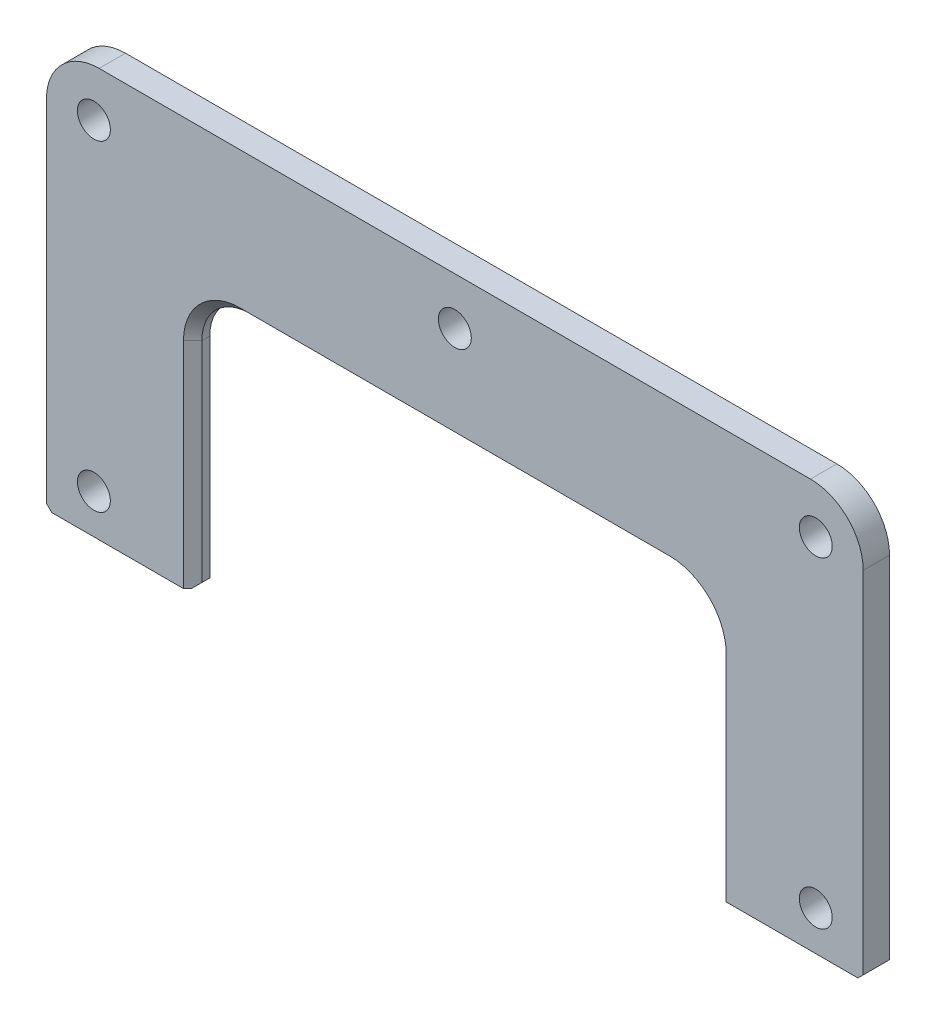
SolidWorks part; units mm, degrees
material "耐油橡胶板 3002"
ref_plane "前视基准面" through (0, 0, 0) normal (0, 0, 1) x (1, 0, 0)
ref_plane "上视基准面" through (0, 0, 0) normal (0, 1, 0) x (1, 0, 0)
ref_plane "右视基准面" through (0, 0, 0) normal (1, 0, 0) x (0, 0, -1)
sketch "草图1" plane through (0, 0, 0) normal (0, 0, 1) x (1, 0, 0)
  line L0 (-155, 0) -> (-99.5, 0)
  line L1 (-81.5, 99.5) -> (81.5, 99.5)
  line L2 (-99.5, 81.5) -> (-99.5, 2.5)
  line L3 (-81.5, -99.5) -> (81.5, -99.5) construction
  line L4 (99.5, 81.5) -> (99.5, 2.5)
  line L5 (-99.5, 99.5) -> (99.5, -99.5) construction
  line L6 (-99.5, -99.5) -> (99.5, 99.5) construction
  line L7 (-135, -155) -> (135, -155) construction
  line L8 (-155, -135) -> (-155, 0) construction
  line L9 (-135, 155) -> (135, 155)
  line L10 (155, -135) -> (155, 0) construction
  line L11 (-155, -155) -> (155, 155) construction
  line L12 (-155, 155) -> (155, -155) construction
  line L13 (-155, 2.5) -> (-99.5, 2.5) construction
  line L14 (-99.5, 2.5) -> (99.5, 2.5) construction
  line L15 (99.5, 2.5) -> (155, 2.5) construction
  line L16 (-155, 2.5) -> (-155, 135)
  line L17 (-99.5, 0) -> (-99.5, -81.5) construction
  line L18 (99.5, 0) -> (99.5, -81.5) construction
  line L19 (155, 2.5) -> (155, 135)
  line L20 (-155, 2.5) -> (-155, 0)
  line L21 (-99.5, 2.5) -> (-99.5, 0)
  line L22 (99.5, 2.5) -> (99.5, 0)
  line L23 (155, 2.5) -> (155, 0)
  line L24 (99.5, 0) -> (155, 0)
  arc A0 (-81.5, -99.5) -> (-99.5, -81.5) centre (-81.5, -81.5) cw construction
  arc A1 (81.5, -99.5) -> (99.5, -81.5) centre (81.5, -81.5) ccw construction
  arc A2 (99.5, 81.5) -> (81.5, 99.5) centre (81.5, 81.5) ccw
  arc A3 (-99.5, 81.5) -> (-81.5, 99.5) centre (-81.5, 81.5) cw
  arc A4 (135, -155) -> (155, -135) centre (135, -135) ccw construction
  arc A5 (-135, -155) -> (-155, -135) centre (-135, -135) cw construction
  arc A6 (155, 135) -> (135, 155) centre (135, 135) ccw
  arc A7 (-155, 135) -> (-135, 155) centre (-135, 135) cw
  point P0 (0, 0)
  point P18 (0, 0)
  dimension "D3" = 18
  dimension "D6" = 20
  dimension "D1" = 199
  dimension "D2" = 199
  dimension "D4" = 310
  dimension "D5" = 310
  dimension "D7" = 2.5
extrude "凸台-拉伸1" add sketch "草图1" along normal blind 10
sketch "草图2" plane through (0, 0, 10) normal (0, 0, 1) x (1, 0, 0)
  line L0 (135, 155) -> (-135, 155) construction
  line L1 (-137, -137) -> (137, -137) construction
  line L2 (-137, -137) -> (-137, 137) construction
  line L3 (-137, 137) -> (137, 137) construction
  line L4 (137, -137) -> (137, 137) construction
  line L5 (-137, -137) -> (137, 137) construction
  line L6 (-137, 137) -> (137, -137) construction
  line L8 (-137, 0) -> (0, 0) construction
  line L9 (0, 0) -> (0, 137) construction
  line L10 (155, 0) -> (155, 135) construction
  circle A0 centre (0, 137) radius 6.25
  circle A1 centre (0, -137) radius 6.25
  circle A2 centre (137, 0) radius 6.25 construction
  circle A3 centre (-137, 0) radius 6.25 construction
  circle A4 centre (-137, 137) radius 6.25
  circle A5 centre (137, 137) radius 6.25
  circle A6 centre (-137, -137) radius 6.25
  circle A7 centre (137, -137) radius 6.25
  circle A8 centre (-137, 15) radius 6.25
  circle A9 centre (-137, -15) radius 6.25
  circle A10 centre (137, -15) radius 6.25
  circle A11 centre (137, 15) radius 6.25
  point P0 (0, 0)
  dimension "D3" = 12.5
  dimension "D1" = 18
  dimension "D2" = 18
  dimension "D4" = 30
extrude "切除-拉伸1" cut sketch "草图2" against normal through all
chamfer "倒角1" distance 2 angle 45 4 edges at (155, 0, 5) (99.5, 0, 5) (-155, 0, 5) (-99.5, 0, 5)
chamfer "倒角2" distance 3.5 angle 45 10 edges at (99.5, 41.75, 0) (94.2279, 94.2279, 0) (0, 99.5, 0) (-94.2279, 94.2279, 0) (-99.5, 41.75, 0) (99.5, 41.75, 10) (94.2279, 94.2279, 10) (-99.5, 41.75, 10) (-94.2279, 94.2279, 10) (0, 99.5, 10)
